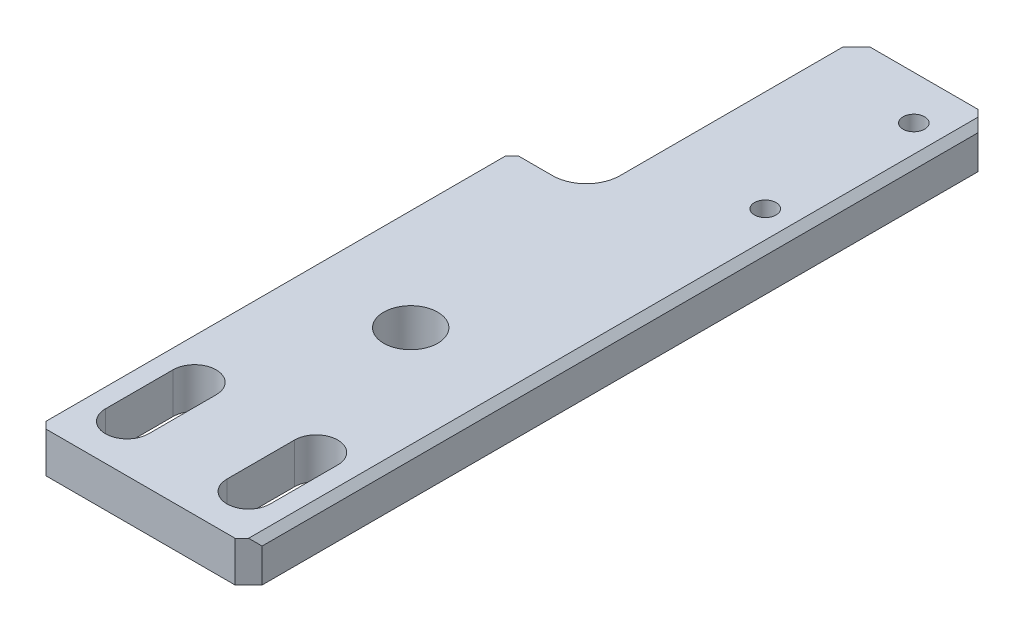
from build123d import *

# Parameters (mm, degrees)
SKETCH1_W                    = 16
SKETCH1_H                    = 55
BOSS_EXTRUDE1_DEPTH          = 3
CUT_EXTRUDE2_DEPTH           = 10
SKETCH5_W                    = 6
SKETCH5_H                    = 20
CUT_EXTRUDE3_DEPTH           = 10
FILLET1_R                    = 2.5
CHAMFER1_SIZE                = 1
CHAMFER2_SIZE                = 0.5
M2_TAPPED_HOLE1_D            = 1.6
M2_TAPPED_HOLE1_DEPTH        = 5.2
M2_TAPPED_HOLE1_TIP          = 0.480688495
F_4_0_4_DIAMETER_HOLE1_D     = 4
F_4_0_4_DIAMETER_HOLE1_DEPTH = 4
F_4_0_4_DIAMETER_HOLE1_TIP   = 1.201721238


with BuildPart() as part:
    # Sketch1 → Boss-Extrude1 (new body)
    with BuildSketch(Plane(origin=(0, 0, 0), x_dir=(1, 0, 0), z_dir=(0, 1, 0))):
        with Locations((8, -27.5)):
            Rectangle(SKETCH1_W, SKETCH1_H)
    extrude(amount=BOSS_EXTRUDE1_DEPTH)

    # Sketch4 → Cut-Extrude2 (cut)
    with BuildSketch(Plane.XZ):
        with BuildLine():
            Line((5.1, 51.5), (5.1, 46.5))
            ThreePointArc((5.1, 46.5), (3.5, 44.9), (1.9, 46.5))
            Line((1.9, 46.5), (1.9, 51.5))
            ThreePointArc((1.9, 51.5), (3.5, 53.1), (5.1, 51.5))
        make_face()
        with BuildLine():
            Line((10.9, 51.5), (10.9, 46.5))
            ThreePointArc((10.9, 46.5), (12.5, 44.9), (14.1, 46.5))
            Line((14.1, 46.5), (14.1, 51.5))
            ThreePointArc((14.1, 51.5), (12.5, 53.1), (10.9, 51.5))
        make_face()
    extrude(amount=-CUT_EXTRUDE2_DEPTH, mode=Mode.SUBTRACT)

    # Sketch5 → Cut-Extrude3 (cut)
    with BuildSketch(Plane(origin=(0, 3, 0), x_dir=(1, 0, 0), z_dir=(0, 1, 0))):
        with Locations((3, -10)):
            Rectangle(SKETCH5_W, SKETCH5_H)
    extrude(amount=-CUT_EXTRUDE3_DEPTH, mode=Mode.SUBTRACT)

    # Fillet1
    fillet1_edges = [part.edges().sort_by_distance(p)[0] for p in [
        (6, 1.5, 20),
    ]]
    fillet(fillet1_edges, radius=FILLET1_R)

    # Chamfer1
    chamfer1_edges = [part.edges().sort_by_distance(p)[0] for p in [
        (0, 1.5, 20),
        (6, 1.5, 0),
        (16, 1.5, 0),
        (16, 1.5, 55),
        (0, 1.5, 55),
    ]]
    chamfer(chamfer1_edges, length=CHAMFER1_SIZE)

    # Chamfer2
    chamfer2_edges = [part.edges().sort_by_distance(p)[0] for p in [
        (0, 3, 37.5),
        (16, 3, 27.5),
    ]]
    chamfer(chamfer2_edges, length=CHAMFER2_SIZE)

    # M2 Tapped Hole1
    with Locations(Plane(origin=(0, 3, 0), x_dir=(1, 0, 0), z_dir=(0, 1, 0))):
        with Locations((13.5, -3.25), (13.5, -14.25)):
            Hole(M2_TAPPED_HOLE1_D / 2, depth=M2_TAPPED_HOLE1_DEPTH)
            with Locations((0, 0, -(M2_TAPPED_HOLE1_DEPTH + M2_TAPPED_HOLE1_TIP / 2))):  # 118° drill point
                Cone(0, M2_TAPPED_HOLE1_D / 2, M2_TAPPED_HOLE1_TIP, mode=Mode.SUBTRACT)

    # Ø4.0 (4) Diameter Hole1
    with Locations(Plane(origin=(0, 0, 0), x_dir=(-1, 0, 0), z_dir=(0, -1, 0))):
        with Locations((-8, -35)):
            Hole(F_4_0_4_DIAMETER_HOLE1_D / 2, depth=F_4_0_4_DIAMETER_HOLE1_DEPTH)
            with Locations((0, 0, -(F_4_0_4_DIAMETER_HOLE1_DEPTH + F_4_0_4_DIAMETER_HOLE1_TIP / 2))):  # 118° drill point
                Cone(0, F_4_0_4_DIAMETER_HOLE1_D / 2, F_4_0_4_DIAMETER_HOLE1_TIP, mode=Mode.SUBTRACT)


solid = part.part
